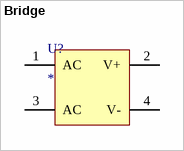
[diagram p0: symbol Bridge]
# Altium schematic symbol library MISC82778-3.SchLib: 1 symbol
Pins are listed as number, name and electrical type; pins without a type are passive.


## Bridge
designator U?
pins: 1 AC, 2 V+, 3 AC, 4 V-